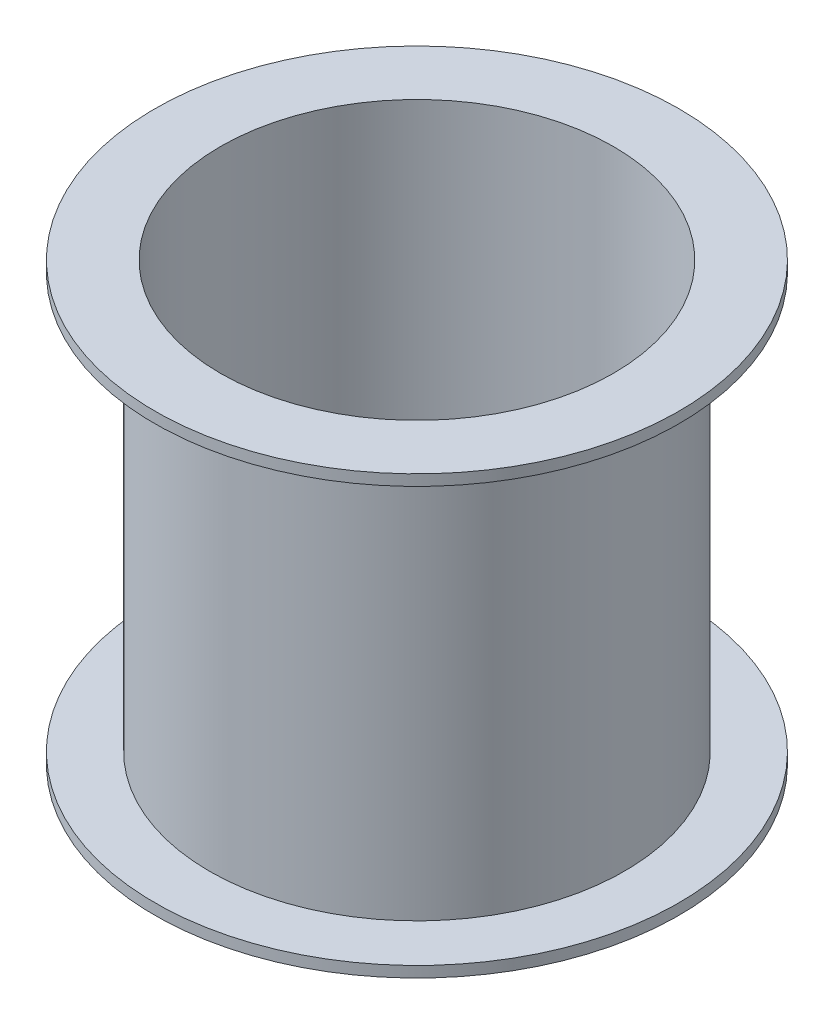
from build123d import *


with BuildPart() as part:
    # Sketch2 → Revolve2 (revolve)
    with BuildSketch(Plane(origin=(0, 0, 0), x_dir=(0, 0, -1), z_dir=(1, 0, 0))):
        Polygon((24, 40), (24, 39), (19, 39), (19, 1), (24, 1), (24, 0), (18, 0), (18, 40), align=None)
    revolve(axis=Axis((0, 0, 0), (0, 1, 0)))


solid = part.part
